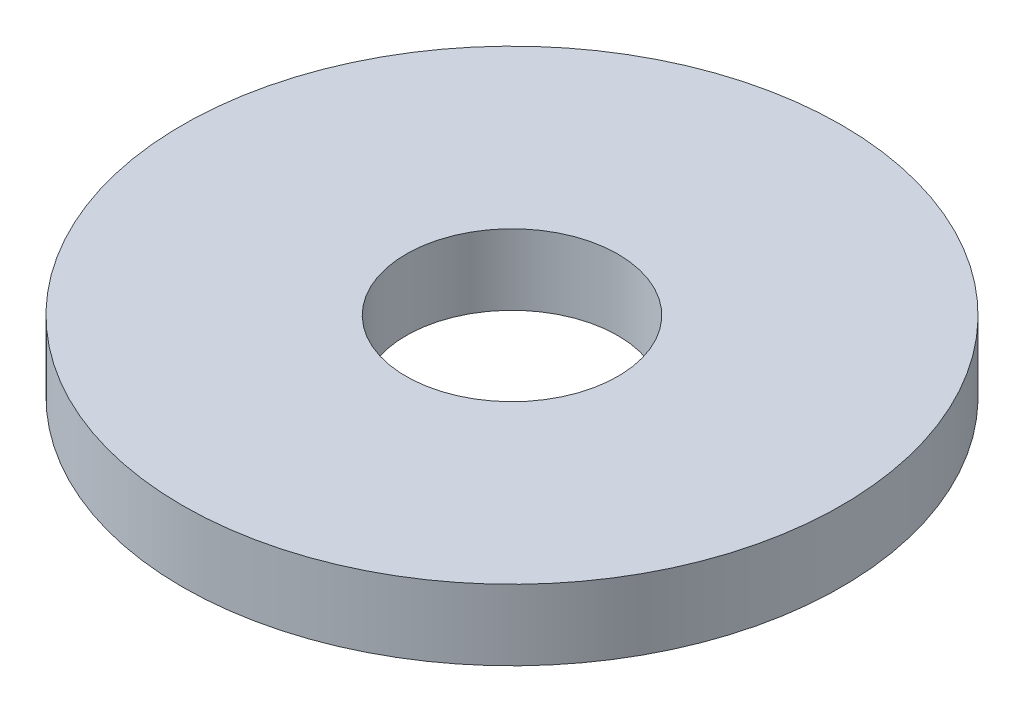
SolidWorks part; units mm, degrees
material "钢"
ref_plane "基准面1" through (0, 0, 0) normal (0, 0, 1) x (1, 0, 0)
ref_plane "基准面2" through (0, 0, 0) normal (0, 1, 0) x (1, 0, 0)
ref_plane "基准面3" through (0, 0, 0) normal (1, 0, 0) x (0, 0, -1)
sketch "尺寸草图" plane through (0, 0, 0) normal (0, 0, 1) x (1, 0, 0)
  line L0 (0, 0) -> (9.1, 0)
  point P3 (3, 0)
  point P4 (28, 0)
  point P5 (9, 0)
sketch "草图1" plane through (0, 0, 0) normal (0, 0, 1) x (1, 0, 0)
  line L0 (0, 0) -> (0, 52.7318) construction
  line L2 (-4.5, 8.6445) -> (-14, 8.6445)
  line L3 (-4.5, 8.6445) -> (-4.5, 11.6445)
  line L4 (-4.5, 11.6445) -> (-14, 11.6445)
  line L5 (-14, 8.6445) -> (-14, 11.6445)
revolve "基体-旋转" add sketch "草图1" angle 360 about L0
equation "\"h@草图1\" = \"h@尺寸草图\""
equation "\"D1@草图1\" = \"d1@尺寸草图\" / 2"
equation "\"D2@草图1\" = \"d2@尺寸草图\" / 2"
